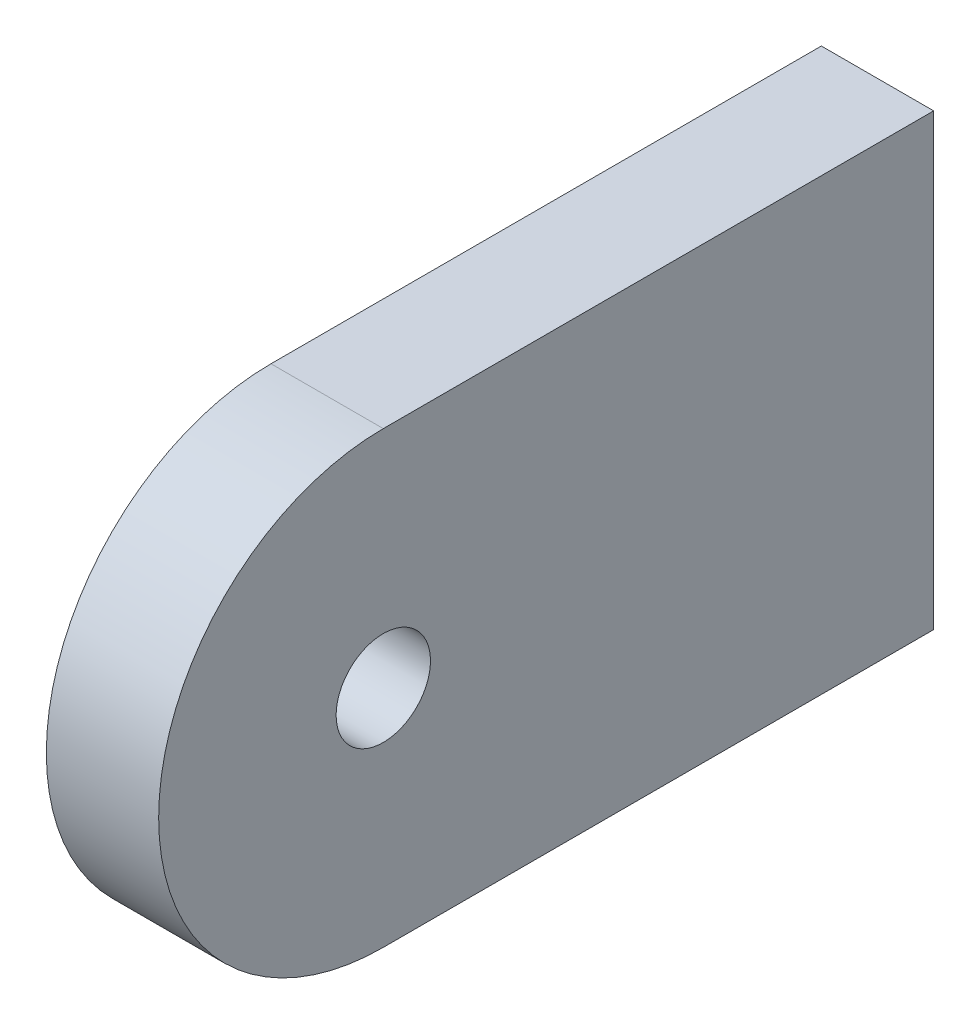
SolidWorks part; units mm, degrees
material "1023 碳钢板 (SS)"
ref_plane "Front Plane" through (0, 0, 0) normal (0, 0, 1) x (1, 0, 0)
ref_plane "Top Plane" through (0, 0, 0) normal (0, 1, 0) x (1, 0, 0)
ref_plane "Right Plane" through (0, 0, 0) normal (1, 0, 0) x (0, 0, -1)
sketch "Sketch1" plane through (0, 0, 0) normal (1, 0, 0) x (0, 0, -1)
  line L1 (-15, 210) -> (-39.5, 210)
  line L2 (-15, 210) -> (-15, 190)
  line L3 (-15, 190) -> (-39.5, 190)
  arc A0 (-39.5, 210) -> (-39.5, 190) centre (-39.5, 200) ccw
  dimension "D1" = 20
extrude "Boss-Extrude1" add sketch "Sketch1" along normal mid plane 5
hole_wizard "M5 Tapped Hole1" positions "3DSketch2" profile "Sketch2" tap size "M5" standard "IS"
sketch3d "3DSketch2"
  line L0 (2.5, 200, 39.5) -> (-2.5, 200, 39.5) construction
  point P0 (-2.5, 200, 39.5)
sketch "Sketch2" plane through (-2.5, 200, 39.5) normal (0, 1, 0) x (0, 0, 1)
  line L0 (0, 0) -> (0, 6.2618)
  line L1 (0, 6.2618) -> (2.1, 5)
  line L2 (2.1, 5) -> (2.1, 0)
  line L5 (2.1, 0) -> (0, 0)
  line L10 (0, 6.2618) -> (-2.1, 5) construction
  line L11 (0, -6.35) -> (0, 107.95) construction
  dimension "螺纹孔钻头直径" = 4.2
  dimension "螺纹孔钻头深度" = 5
  dimension "导头角度" = 118
cosmetic thread "Cosmetic thread 1" parameters "D1"=5, "D2"=5
